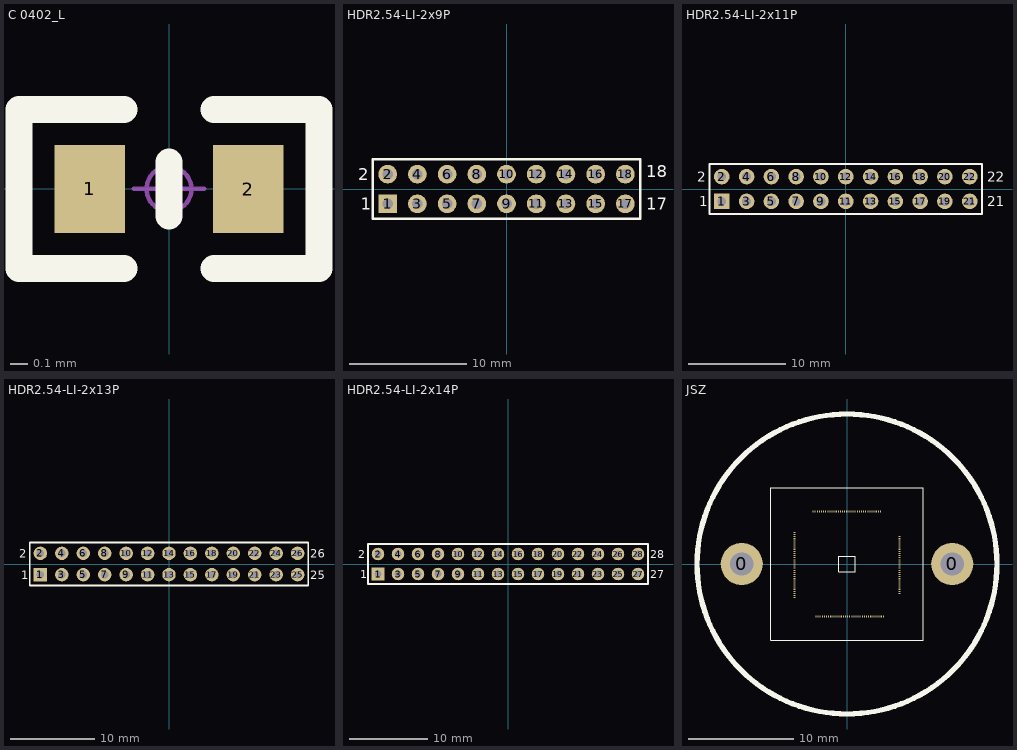
[diagram p0: the footprints below, top view; thin cyan lines are the x and y axes]
# Altium footprint library MISC82784.PcbLib: 6 footprints
Each footprint in its own frame and in the unit in brackets; x right, y up, seen from the top. Pads: shape width x height; smd on the part's side, far side on the other; paste and mask are expansions set on the pad; w line width, h text height; cw(c..) or ccw(c..) is an arc to the next point about the centre after c.

## C 0402_L [mm]
pads (2):
  rect 0.4x0.5 smd: 1(-0.45,0) 2(0.45,0)
Top Overlay:
  lines w0.152: -0.254,-0.45 -0.85,-0.45 ; -0.254,0.45 -0.85,0.45 -0.85,-0.45 ; 0,-0.152 0,0.152 ; 0.254,-0.45 0.85,-0.45 0.85,0.45 0.254,0.45 ; -0.85,-0.45 -0.85,-0.45
Mechanical 15:
  circle w0.025: c0,0 r0.127
  lines w0.025: -0.2,0 0.2,0 ; 0,-0.2 0,0.2

## HDR2.54-LI-2x9P [mm]
pads (18):
  rect 1.6x1.6 hole 0.9: 1(-10.16,-1.27)
  round 1.6 hole 0.9: 2(-10.16,1.27) 3(-7.62,-1.27) 4(-7.62,1.27) 5(-5.08,-1.27) 6(-5.08,1.27) 7(-2.54,-1.27) 8(-2.54,1.27) 9(0,-1.27) 10(0,1.27) 11(2.54,-1.27) 12(2.54,1.27) 13(5.08,-1.27) 14(5.08,1.27) 15(7.62,-1.27) 16(7.62,1.27) 17(10.16,-1.27) 18(10.16,1.27)
Top Overlay:
  lines w0.2: -11.43,-2.54 11.43,-2.54 11.43,2.54 -11.43,2.54 -11.43,-2.54
  text "17" at 11.938,-1.778 h1.02
  text "18" at 11.938,1.016 h1.02
  text "1" at -12.446,-1.778 h1.02
  text "2" at -12.7,0.762 h1.02

## HDR2.54-LI-2x11P [mm]
pads (22):
  rect 1.6x1.6 hole 0.9: 1(-12.7,-1.27)
  round 1.6 hole 0.9: 2(-12.7,1.27) 3(-10.16,-1.27) 4(-10.16,1.27) 5(-7.62,-1.27) 6(-7.62,1.27) 7(-5.08,-1.27) 8(-5.08,1.27) 9(-2.54,-1.27) 10(-2.54,1.27) 11(0,-1.27) 12(0,1.27) 13(2.54,-1.27) 14(2.54,1.27) 15(5.08,-1.27) 16(5.08,1.27) 17(7.62,-1.27) 18(7.62,1.27) 19(10.16,-1.27) 20(10.16,1.27) 21(12.7,-1.27) 22(12.7,1.27)
Top Overlay:
  lines w0.2: -13.97,-2.54 13.97,-2.54 13.97,2.54 -13.97,2.54 -13.97,-2.54
  text "22" at 14.478,0.762 h1.02
  text "21" at 14.478,-1.778 h1.02
  text "2" at -15.24,0.762 h1.02
  text "1" at -14.986,-1.778 h1.02

## HDR2.54-LI-2x13P [mm]
pads (26):
  rect 1.6x1.6 hole 0.9: 1(-15.24,-1.27)
  round 1.6 hole 0.9: 2(-15.24,1.27) 3(-12.7,-1.27) 4(-12.7,1.27) 5(-10.16,-1.27) 6(-10.16,1.27) 7(-7.62,-1.27) 8(-7.62,1.27) 9(-5.08,-1.27) 10(-5.08,1.27) 11(-2.54,-1.27) 12(-2.54,1.27) 13(0,-1.27) 14(0,1.27) 15(2.54,-1.27) 16(2.54,1.27) 17(5.08,-1.27) 18(5.08,1.27) 19(7.62,-1.27) 20(7.62,1.27) 21(10.16,-1.27) 22(10.16,1.27) 23(12.7,-1.27) 24(12.7,1.27) 25(15.24,-1.27) 26(15.24,1.27)
Top Overlay:
  lines w0.2: -16.51,-2.54 16.51,-2.54 16.51,2.54 -16.51,2.54 -16.51,-2.54
  text "26" at 16.764,0.762 h1.02
  text "25" at 16.764,-1.778 h1.02
  text "1" at -17.526,-1.778 h1.02
  text "2" at -17.78,0.762 h1.02

## HDR2.54-LI-2x14P [mm]
pads (28):
  rect 1.6x1.6 hole 0.9: 1(-16.51,-1.27)
  round 1.6 hole 0.9: 2(-16.51,1.27) 3(-13.97,-1.27) 4(-13.97,1.27) 5(-11.43,-1.27) 6(-11.43,1.27) 7(-8.89,-1.27) 8(-8.89,1.27) 9(-6.35,-1.27) 10(-6.35,1.27) 11(-3.81,-1.27) 12(-3.81,1.27) 13(-1.27,-1.27) 14(-1.27,1.27) 15(1.27,-1.27) 16(1.27,1.27) 17(3.81,-1.27) 18(3.81,1.27) 19(6.35,-1.27) 20(6.35,1.27) 21(8.89,-1.27) 22(8.89,1.27) 23(11.43,-1.27) 24(11.43,1.27) 25(13.97,-1.27) 26(13.97,1.27) 27(16.51,-1.27) 28(16.51,1.27)
Top Overlay:
  lines w0.2: -17.78,-2.54 -17.78,2.54 17.78,2.54 17.78,-2.54 -17.78,-2.54
  text "2" at -19.05,0.762 h1.02
  text "1" at -18.796,-1.778 h1.02
  text "27" at 18.034,-1.778 h1.02
  text "28" at 18.034,0.762 h1.02

## JSZ [mm]
pads (128):
  round 4 hole 2.2: 0(-10,0) 0(10,0)
  rect 0.1x0.2 smd: 1(3.177,5) 2(2.977,5) 3(2.777,5) 4(2.577,5) 5(2.377,5) 6(2.177,5) 7(1.977,5) 8(1.777,5) 9(1.577,5) 10(1.377,5) 11(1.177,5) 12(0.977,5) 13(0.777,5) 14(0.577,5) 15(0.377,5) 16(0.177,5) 17(-0.023,5) 18(-0.223,5) 19(-0.423,5) 20(-0.623,5) 21(-0.823,5) 22(-1.023,5) 23(-1.223,5) 24(-1.423,5) 25(-1.623,5) 26(-1.823,5) 27(-2.023,5) 28(-2.223,5) 29(-2.423,5) 30(-2.623,5) 31(-2.823,5) 32(-3.023,5) 33(-3.223,5) 66(-2.946,-5) 67(-2.746,-5) 68(-2.546,-5) 69(-2.346,-5) 70(-2.146,-5) 71(-1.946,-5) 72(-1.746,-5) 73(-1.546,-5) 74(-1.346,-5) 75(-1.146,-5) 76(-0.946,-5) 77(-0.746,-5) 78(-0.546,-5) 79(-0.346,-5) 80(-0.146,-5) 81(0.054,-5) 82(0.254,-5) 83(0.454,-5) 84(0.654,-5) 85(0.854,-5) 86(1.054,-5) 87(1.254,-5) 88(1.454,-5) 89(1.654,-5) 90(1.854,-5) 91(2.054,-5) 92(2.254,-5) 93(2.454,-5) 94(2.654,-5) 95(2.854,-5) 96(3.054,-5) 97(3.254,-5) 98(3.454,-5)
  rect 0.2x0.1 smd: 34(-5,3) 35(-5,2.8) 36(-5,2.6) 37(-5,2.4) 38(-5,2.2) 39(-5,2) 40(-5,1.8) 41(-5,1.6) 42(-5,1.4) 43(-5,1.2) 44(-5,1) 45(-5,0.8) 46(-5,0.6) 47(-5,0.4) 48(-5,0.2) 49(-5,0) 50(-5,-0.2) 51(-5,-0.4) 52(-5,-0.6) 53(-5,-0.8) 54(-5,-1) 55(-5,-1.2) 56(-5,-1.4) 57(-5,-1.6) 58(-5,-1.8) 59(-5,-2) 60(-5,-2.2) 61(-5,-2.4) 62(-5,-2.6) 63(-5,-2.8) 64(-5,-3) 65(-5,-3.2) 99(5,-2.8) 100(5,-2.6) 101(5,-2.4) 102(5,-2.2) 103(5,-2) 104(5,-1.8) 105(5,-1.6) 106(5,-1.4) 107(5,-1.2) 108(5,-1) 109(5,-0.8) 110(5,-0.6) 111(5,-0.4) 112(5,-0.2) 113(5,0) 114(5,0.2) 115(5,0.4) 116(5,0.6) 117(5,0.8) 118(5,1) 119(5,1.2) 120(5,1.4) 121(5,1.6) 122(5,1.8) 123(5,2) 124(5,2.2) 125(5,2.4) 126(5,2.6)
Top Overlay:
  circle w0.5: c0,0 r14.25
  lines w0.1: -7.25,-7.25 7.25,-7.25 7.25,7.25 -7.25,7.25 -7.25,-7.25 ; -0.8,-0.75 -0.8,0.75 0.8,0.75 0.8,-0.75 -0.8,-0.75